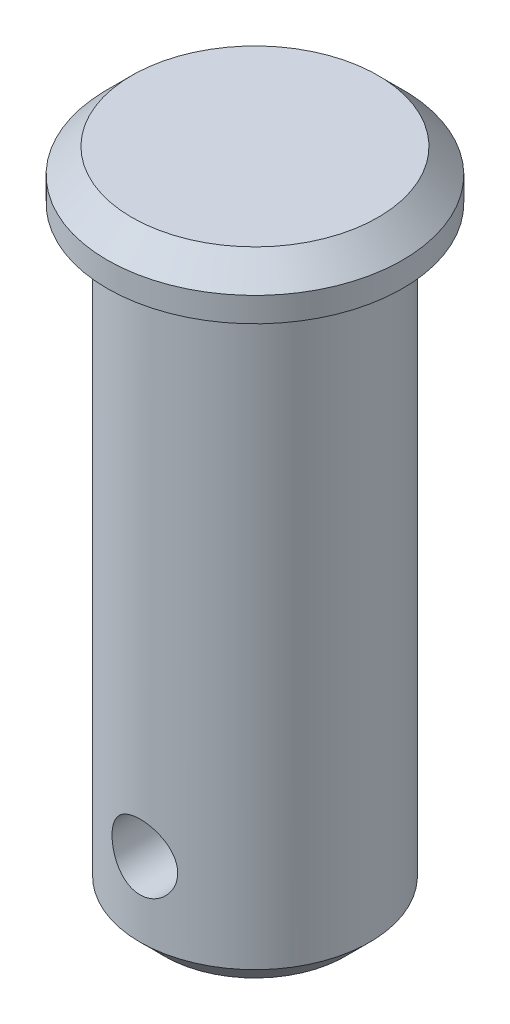
from build123d import *

# Parameters (mm, degrees)
SKETCH_1_R               = 9
EXTRUDE_1_DEPTH          = 3
SKETCH_2_R               = 7
EXTRUDE_2_DEPTH          = 37
CHAMFER_1_SIZE           = 1.5
CUT_EXTRUDE_2_DEPTH      = 40.127995093
CUT_EXTRUDE_2_DEPTH_BACK = 40.127995093
SKETCH_10_R              = 2
FILLET_1_R               = 0.5


with BuildPart() as part:
    # 草图1 → 凸台-拉伸1 (new body)
    with BuildSketch(Plane(origin=(0, 0, 0), x_dir=(1, 0, 0), z_dir=(0, 1, 0))):
        with Locations(Location((0, 0, 0), (0, 0, 270))):
            Circle(SKETCH_1_R)
    extrude(amount=EXTRUDE_1_DEPTH)

    # 草图2 → 凸台-拉伸2 (add)
    with BuildSketch(Plane.XZ):
        with Locations(Location((0, 0, 0), (0, 0, 270))):
            Circle(SKETCH_2_R)
    extrude(amount=EXTRUDE_2_DEPTH)

    # 倒角1
    chamfer_1_edges = [part.edges().sort_by_distance(p)[0] for p in [
        (0, 3, -9),
        (0, -37, 7),
    ]]
    chamfer(chamfer_1_edges, length=CHAMFER_1_SIZE)

    # 草图10 → 切除-拉伸2 (cut, two sides: drawn at the far end of the back side and taken through both)
    with BuildSketch(Plane.XY.offset(-CUT_EXTRUDE_2_DEPTH_BACK)):
        with Locations(Location((0, -31, 0), (0, 0, 270.00000003))):
            Circle(SKETCH_10_R)
    extrude(amount=CUT_EXTRUDE_2_DEPTH + CUT_EXTRUDE_2_DEPTH_BACK, mode=Mode.SUBTRACT)

    # 圆角1
    fillet_1_edges = [part.edges().sort_by_distance(p)[0] for p in [
        (0, 0, 7),
    ]]
    fillet(fillet_1_edges, radius=FILLET_1_R)


solid = part.part
